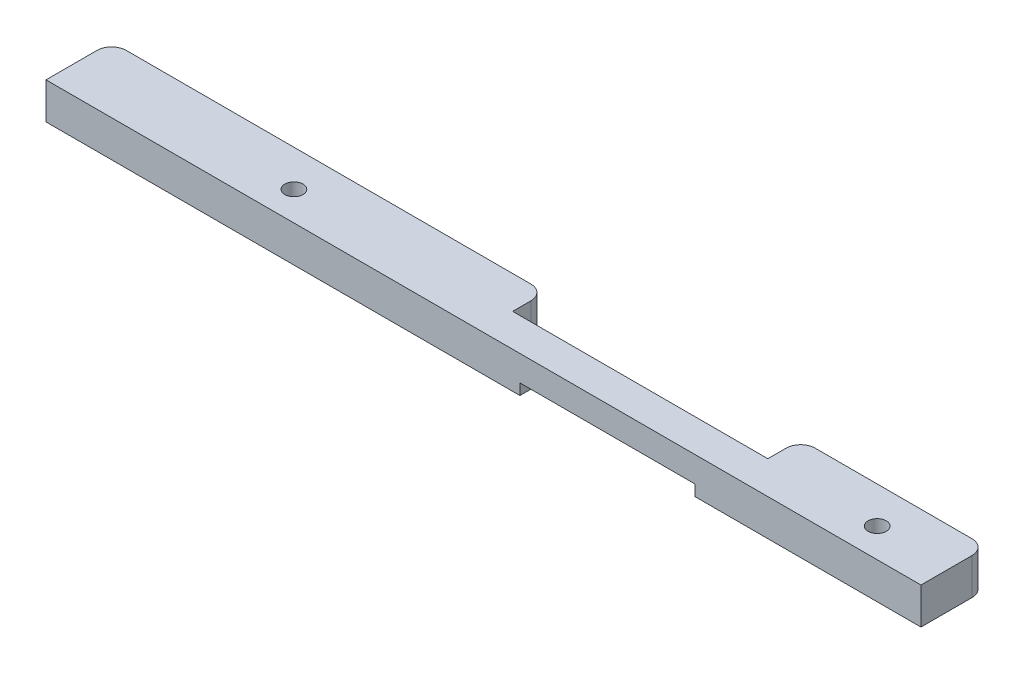
SolidWorks part; units mm, degrees
ref_plane "Front Plane" through (0, 0, 0) normal (0, 0, 1) x (1, 0, 0)
ref_plane "Top Plane" through (0, 0, 0) normal (0, 1, 0) x (1, 0, 0)
ref_plane "Right Plane" through (0, 0, 0) normal (1, 0, 0) x (0, 0, -1)
sketch "Sketch1" plane through (0, 0, 0) normal (0, 1, 0) x (1, 0, 0)
  line L0 (0, 0) -> (0, 9)
  line L1 (0, 9) -> (120, 9)
  line L2 (120, 9) -> (120, 0)
  line L3 (120, 0) -> (0, 0)
  dimension "D1" = 9
  dimension "D2" = 120
extrude "Boss-Extrude1" add sketch "Sketch1" along normal blind 5
hole_wizard "M3 Tapped Hole1" positions "Sketch3" profile "Sketch2" tap size "M3" standard "GB"
sketch "Sketch3" plane through (0, 5, 0) normal (0, 1, 0) x (-1, 0, 0)
  line L0 (0, -9) -> (0, 0) construction
  line L2 (0, 0) -> (-120, 0) construction
  point P0 (-30, -4)
  point P1 (-110, -4)
  dimension "D1" = 80
  dimension "D2" = 30
  dimension "D3" = 4
sketch "Sketch2" plane through (30, 5, -4) normal (1, 0, 0) x (0, 0, 1)
  line L0 (0, 0) -> (0, 8.5)
  line L1 (0, 8.5) -> (1.25, 8.5)
  line L2 (1.25, 8.5) -> (1.25, 0)
  line L5 (1.25, 0) -> (0, 0)
  line L10 (0, 8.5) -> (-1.25, 8.5) construction
  line L11 (0, -6.35) -> (0, 107.95) construction
  dimension "螺纹孔钻头直径" = 2.5
  dimension "螺纹孔钻头深度" = 8.5
  dimension "导头角度" = 180
cosmetic thread "Cosmetic Thread2" parameters "D1"=5, "D2"=3
cosmetic thread "Cosmetic Thread3" parameters "D1"=5, "D2"=3
sketch "Sketch4" plane through (0, 5, 0) normal (0, 1, 0) x (-1, 0, 0)
  line L0 (-120, -9) -> (0, -9) construction
  line L1 (-94.5, -9) -> (-59.5, -9)
  line L2 (-94.5, -9) -> (-94.5, -4.5)
  line L3 (-94.5, -4.5) -> (-59.5, -4.5)
  line L4 (-59.5, -9) -> (-59.5, -4.5)
  line L5 (-120, 0) -> (-120, -9) construction
  dimension "D1" = 4.5
  dimension "D2" = 25.5
  dimension "D3" = 35
fillet "Fillet1" radius 2 2 edges at (0, 2.5, -9) (120, 2.5, -9)
extrude "Cut-Extrude1" cut sketch "Sketch4" against normal through all
fillet "Fillet2" radius 2 2 edges at (94.5, 2.5, -9) (59.5, 2.5, -9)
sketch "Sketch5" plane through (0, 0, 0) normal (0, -1, 0) x (1, 0, 0)
  line L0 (59.5, -4.5) -> (94.5, -4.5) construction
  line L1 (89, -9) -> (65, -9)
  line L2 (89, -9) -> (89, 0)
  line L3 (89, 0) -> (65, 0)
  line L4 (65, -9) -> (65, 0)
  line L5 (89, -9) -> (65, 0) construction
  line L6 (89, 0) -> (65, -9) construction
  line L7 (0, 0) -> (120, 0) construction
  point P0 (77, -4.5)
  dimension "D1" = 24
extrude "Cut-Extrude2" cut sketch "Sketch5" against normal blind 1.5
